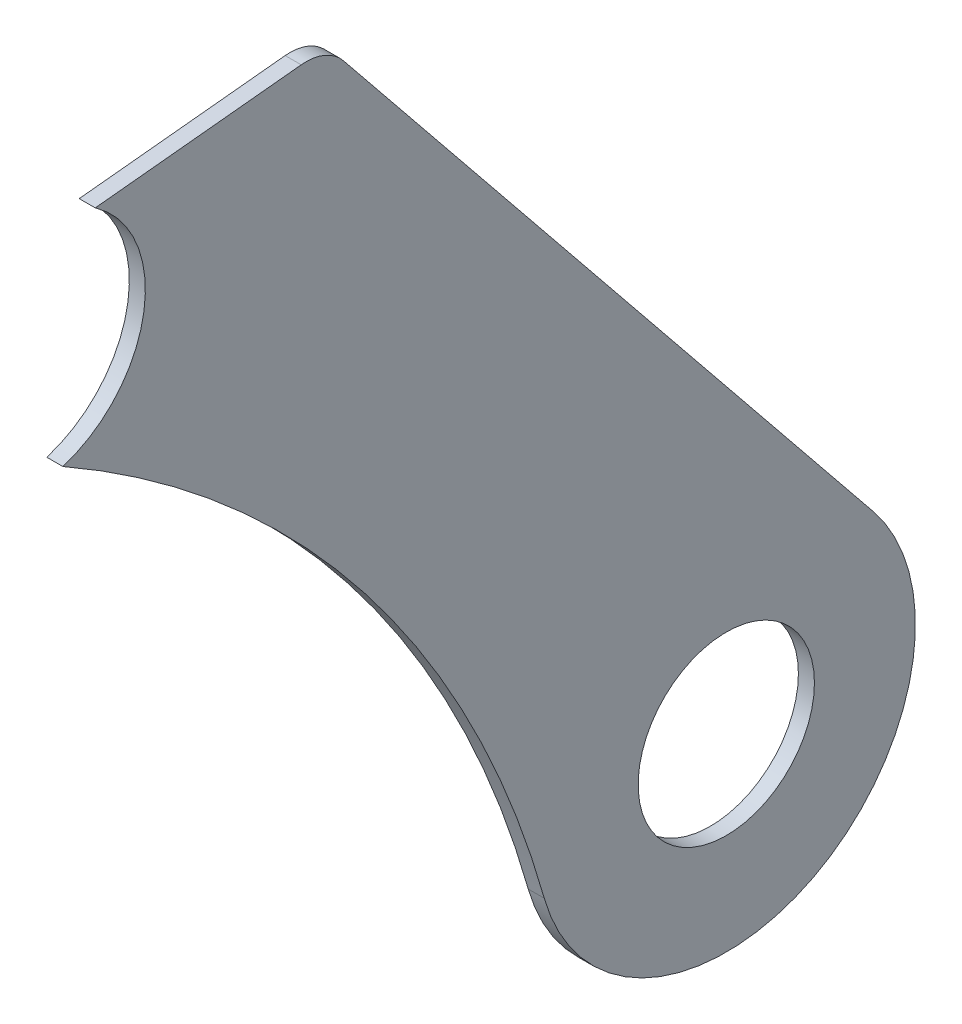
SolidWorks part; units mm, degrees
ref_plane "Front Plane" through (0, 0, 0) normal (0, 0, 1) x (1, 0, 0)
ref_plane "Top Plane" through (0, 0, 0) normal (0, 1, 0) x (1, 0, 0)
ref_plane "Right Plane" through (0, 0, 0) normal (1, 0, 0) x (0, 0, -1)
sketch "Sketch1" plane through (0, 0, 0) normal (1, 0, 0) x (0, 0, -1)
  line L0 (337.6252, 687.7) -> (466.147, 700.7587)
  line L1 (492.5082, 689.7744) -> (823.1745, 280.8025)
  arc A0 (617.8247, 174.5182) -> (317.4153, 558.0426) centre (0, 0) ccw
  arc A1 (617.8247, 174.5182) -> (823.1745, 280.8025) centre (731.4, 206.6) ccw
  circle A2 centre (731.4, 206.6) radius 55
  arc A3 (317.4153, 558.0426) -> (337.6252, 687.7) centre (295.9, 627.8) ccw
  arc A4 (466.147, 700.7587) -> (492.5082, 689.7744) centre (469.1796, 670.9124) cw
  point P10 (482.3, 702.4)
  dimension "D1" = 1284
  dimension "D4" = 110
  dimension "D7" = 146
  dimension "D11" = 30
  dimension "D2" = 731.4
  dimension "D3" = 206.6
  dimension "D5" = 421.2
  dimension "D6" = 435.5
  dimension "D8" = 59.9
  dimension "D9" = 74.6
  dimension "D10" = 186.4
extrude "Boss-Extrude1" add sketch "Sketch1" along normal blind 10
